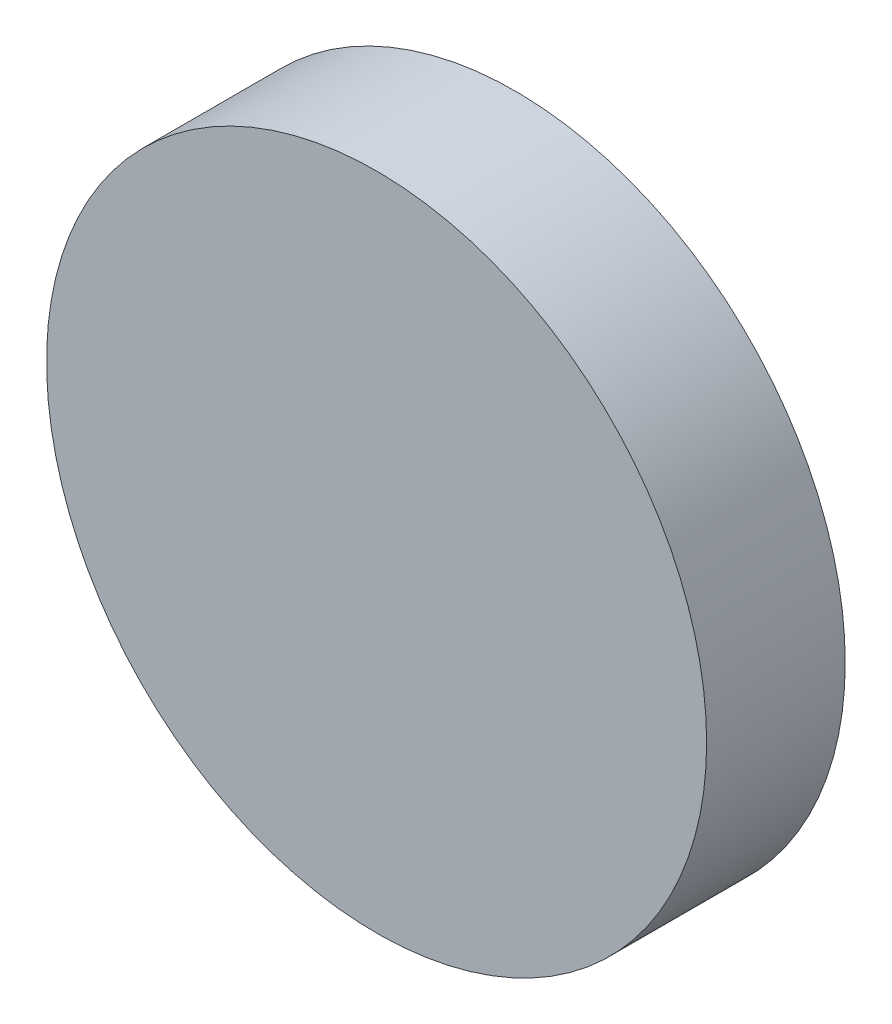
SolidWorks part; units mm, degrees
ref_plane "Front" through (0, 0, 0) normal (0, 0, 1) x (1, 0, 0)
ref_plane "Top" through (0, 0, 0) normal (0, 1, 0) x (1, 0, 0)
ref_plane "Right" through (0, 0, 0) normal (1, 0, 0) x (0, 0, -1)
sketch "Sketch1" plane through (0, 0, 0) normal (0, 0, 1) x (1, 0, 0)
  circle A0 centre (0, 0) radius 250
  dimension "D1" = 500
extrude "Boss-Extrude1" add sketch "Sketch1" along normal blind 105
